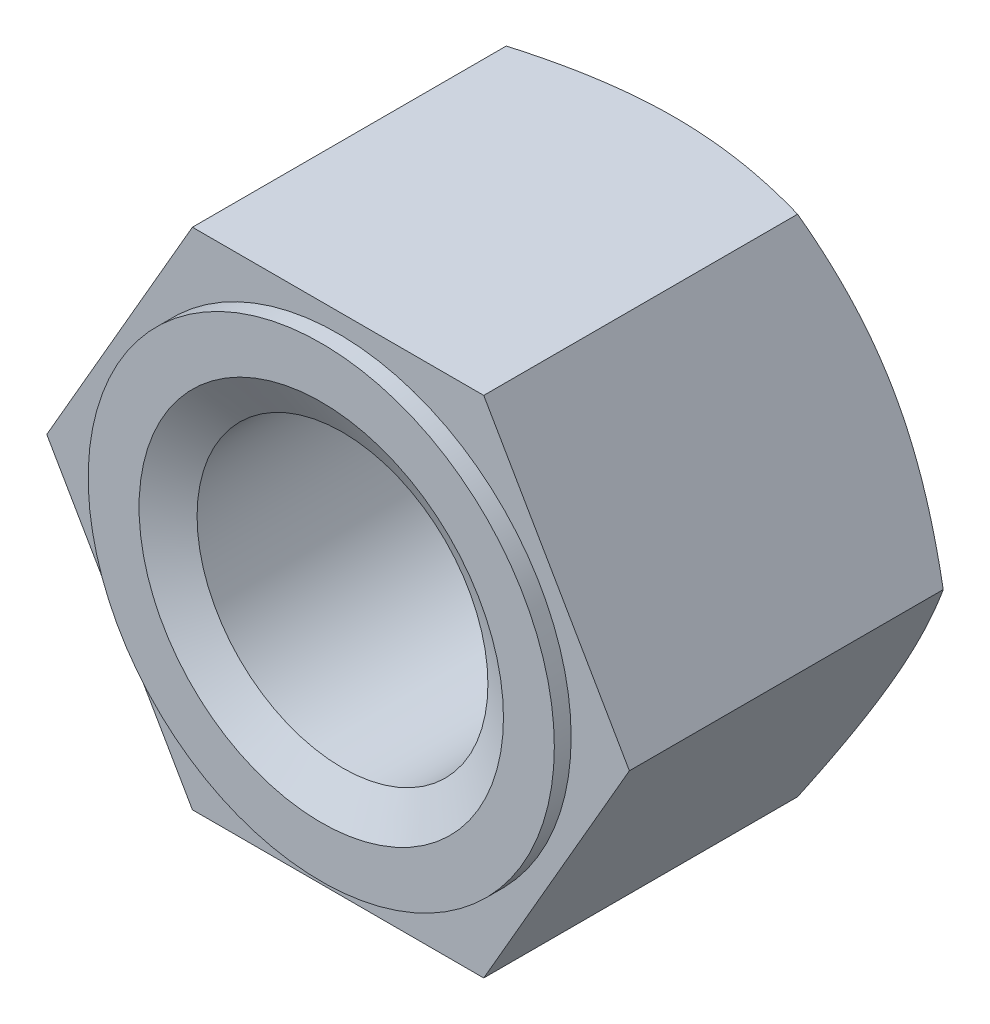
SolidWorks part; units mm, degrees
ref_plane "Front" through (0, 0, 0) normal (0, 0, 1) x (1, 0, 0)
ref_plane "Top" through (0, 0, 0) normal (0, 1, 0) x (1, 0, 0)
ref_plane "Right" through (0, 0, 0) normal (1, 0, 0) x (0, 0, -1)
other "Configuration Table"
sketch "Sketch1" plane through (0, 0, 0) normal (0, 0, 1) x (1, 0, 0)
  line L1 (5.1962, -9) -> (10.3923, 0)
  line L2 (10.3923, 0) -> (5.1962, 9)
  line L3 (5.1962, 9) -> (-5.1962, 9)
  line L4 (-5.1962, 9) -> (-10.3923, 0)
  line L5 (-10.3923, 0) -> (-5.1962, -9)
  line L6 (-5.1962, -9) -> (5.1962, -9)
  circle A0 centre (0, 0) radius 9 construction
  circle A1 centre (0, 0) radius 5.188
extrude "BaseNut" add sketch "Sketch1" against normal blind 12
cosmetic thread "ThreadCosmetic1" parameters "D2"=13
sketch "Sketch2" plane through (-16.7061, 0, -15.0481) normal (0, 1, 0) x (0, 0, 1)
  line L0 (-23.7227, 16.7061) -> (22.0646, 16.7061) construction
  line L2 (3.0481, 25.7061) -> (3.0481, 27.0985)
  line L4 (3.0481, 27.0985) -> (3.852, 27.0985)
  line L6 (3.852, 27.0985) -> (3.0481, 25.7061)
revolve "Chamfer1" cut sketch "Sketch2" angle 360 about L0
sketch "Sketch6" plane through (-9.1975, 0, -10.2525) normal (0, 1, 0) x (0, 0, 1)
  line L0 (23.3574, 9.1975) -> (-22.3023, 9.1975) construction
  line L2 (-1.7475, 14.3855) -> (-1.7475, 15.6975)
  line L4 (-1.7475, 15.6975) -> (-0.99, 14.3855)
  line L6 (-0.99, 14.3855) -> (-1.7475, 14.3855)
revolve "EndChamfer1" cut sketch "Sketch6" angle 360 about L0
sketch "Sketch5" plane through (-14.793, 0, -16.9612) normal (0, 1, 0) x (0, 0, 1)
  line L0 (-22.5748, 14.793) -> (24.743, 14.793) construction
  line L2 (16.9612, 23.108) -> (16.9612, 25.1853)
  line L4 (16.9612, 25.1853) -> (15.7619, 25.1853)
  line L6 (15.7619, 25.1853) -> (16.9612, 23.108)
  dimension "dw1" = 16.63
  dimension "D2" = 30
revolve "Chamfer2" [suppressed] cut sketch "Sketch5" angle 360 about L0
sketch "Sketch3" plane through (-18.4892, 11.179, 0) normal (0, 0, 1) x (1, 0, 0)
  circle A1 centre (18.4892, -11.179) radius 5.188 construction
  circle A2 centre (18.4892, -11.179) radius 8.315
  circle A3 centre (18.4892, -11.179) radius 5.188
  dimension "dw" = 16.63
extrude "Extrude1" add sketch "Sketch3" along normal blind 0.6
chamfer "EndChamfer3" distance 1.312 angle 30 1 edges at (5.188, 0, 0.6)
chamfer "EndChamfer2" [suppressed] distance 0.4 angle 45
sketch "Sketch7" plane through (0, 0, 0) normal (0, 1, 0) x (1, 0, 0)
  line L0 (0, 61.6098) -> (0, -22.305) construction
  line L1 (3.876, 11.8985) -> (5.188, 11.8985)
  line L2 (5.188, 11.8985) -> (6.3242, 11.2425)
  line L3 (6.3242, 11.2425) -> (5.188, 10.5865)
  line L4 (5.188, 10.5865) -> (3.876, 10.5865)
  line L5 (3.876, 10.5865) -> (3.876, 11.8985)
  line L6 (5.188, 11.2425) -> (-5.188, 11.2425) construction
revolve "Cut-Revolve10" [suppressed] cut sketch "Sketch7" angle 360 about L0
pattern_linear "LPattern10" [suppressed] count 8 spacing 1.5744 along (0, 0, 1)
equation "\"D1@EndChamfer3\" = ( \"da@Sketch6\" - \"D1@Sketch1\" )  / 2"
equation "\"D1@EndChamfer2\" = \"m@BaseNut\" / 30"
equation "\"S1@Sketch2\" = \"s@Sketch1\""
equation "\"D2@Sketch7\" = \"D1@Sketch1\""
equation "\"D1@Sketch7\" = (  \"D2@ThreadCosmetic1\" - \"D1@Sketch1\" )  / 2"
equation "\"D3@LPattern10\" = \"D1@Sketch7\" * 1.2"
equation "\"D1@LPattern10\" =  \"m@BaseNut\"  / \"D3@LPattern10\""
